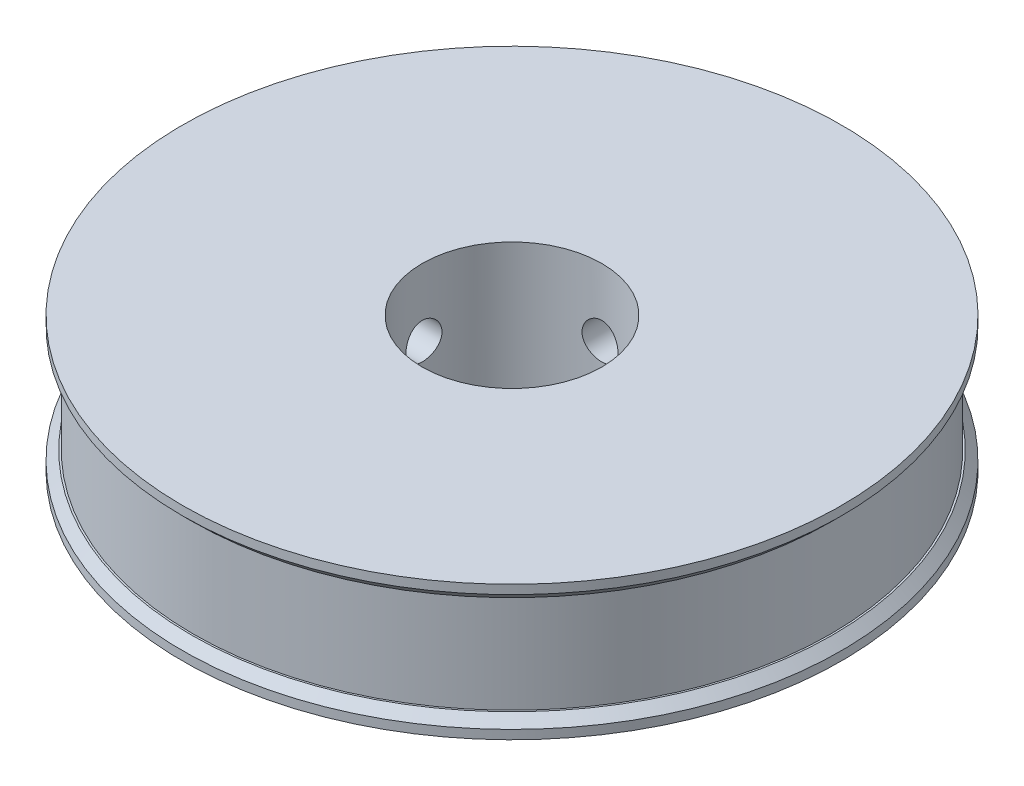
from build123d import *

# Parameters (mm, degrees)
SKETCH1_R           = 35.5
SKETCH1_R_2         = 10
BOSS_EXTRUDE1_DEPTH = 11
SKETCH2_R           = 36.7
SKETCH2_R_2         = 10
BOSS_EXTRUDE2_DEPTH = 2
BOSS_EXTRUDE3_START = 2
SKETCH3_R           = 36.7
SKETCH3_R_2         = 10
BOSS_EXTRUDE3_DEPTH = 2
CHAMFER1_SIZE       = 1
SKETCH5_R           = 2
CUT_EXTRUDE1_DEPTH  = 43
SKETCH6_R           = 2
CUT_EXTRUDE2_DEPTH  = 43


with BuildPart() as part:
    # Sketch1 → Boss-Extrude1 (new body)
    with BuildSketch(Plane(origin=(0, 0, 0), x_dir=(1, 0, 0), z_dir=(0, 1, 0))):
        with Locations(Location((0, 0, 0), (0, 0, 270))):
            Circle(SKETCH1_R)
        with Locations(Location((0, 0, 0), (0, 0, 270))):
            Circle(SKETCH1_R_2, mode=Mode.SUBTRACT)
    extrude(amount=BOSS_EXTRUDE1_DEPTH)

    # Sketch2 → Boss-Extrude2 (add)
    with BuildSketch(Plane(origin=(0, 11, 0), x_dir=(1, 0, 0), z_dir=(0, 1, 0))):
        with Locations(Location((0, 0, 0), (0, 0, 270))):
            Circle(SKETCH2_R)
        with Locations(Location((0, 0, 0), (0, 0, 270))):
            Circle(SKETCH2_R_2, mode=Mode.SUBTRACT)
    extrude(amount=BOSS_EXTRUDE2_DEPTH)

    # Sketch3 → Boss-Extrude3 (add)
    with BuildSketch(Plane.XZ.offset(BOSS_EXTRUDE3_START)):
        with Locations(Location((0, 0, 0), (0, 0, 90))):
            Circle(SKETCH3_R)
        with Locations(Location((0, 0, 0), (0, 0, 270))):
            Circle(SKETCH3_R_2, mode=Mode.SUBTRACT)
    extrude(amount=-BOSS_EXTRUDE3_DEPTH)

    # Chamfer1
    chamfer1_edges = [part.edges().sort_by_distance(p)[0] for p in [
        (0, 11, -36.7),
        (0, 0, -36.7),
    ]]
    chamfer(chamfer1_edges, length=CHAMFER1_SIZE)

    # Sketch5 → Cut-Extrude1 (cut)
    with BuildSketch(Plane.XY):
        with Locations(Location((0, 5.5, 0), (0, 0, 90))):
            Circle(SKETCH5_R)
    extrude(amount=-CUT_EXTRUDE1_DEPTH, mode=Mode.SUBTRACT)

    # Sketch6 → Cut-Extrude2 (cut)
    with BuildSketch(Plane(origin=(0, 0, 0), x_dir=(0, 0, -1), z_dir=(1, 0, 0))):
        with Locations((0, 5.5)):
            Circle(SKETCH6_R)
    extrude(amount=-CUT_EXTRUDE2_DEPTH, mode=Mode.SUBTRACT)


solid = part.part
